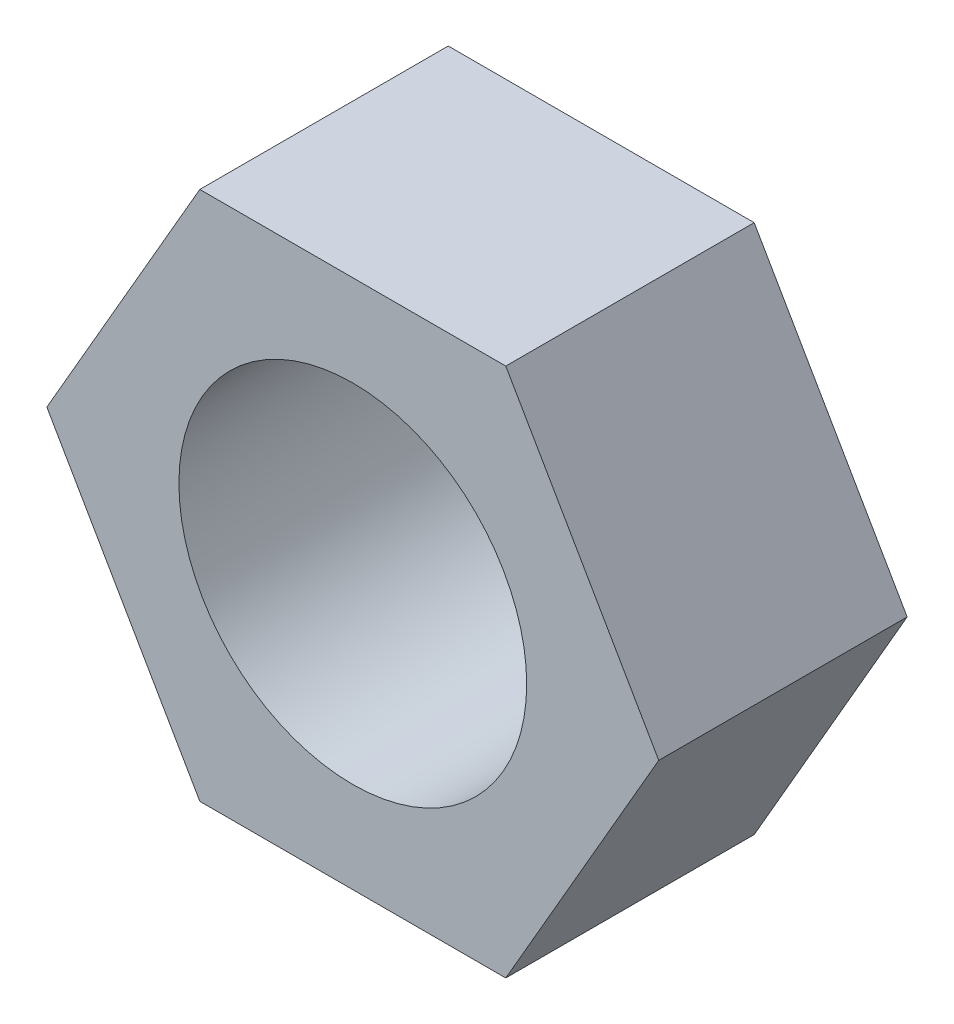
from build123d import *

# Parameters (mm, degrees)
BOSS_EXTRUDE1_DEPTH    = 15
M24_TAPPED_HOLE1_D     = 21
M24_TAPPED_HOLE1_DEPTH = 57
M24_TAPPED_HOLE1_TIP   = 6.3090365


with BuildPart() as part:
    # Sketch1 → Boss-Extrude1 (new body)
    with BuildSketch(Plane.XY):
        Polygon((18.475208614, 0), (9.237604307, 16), (-9.237604307, 16), (-18.475208614, 0), (-9.237604307, -16), (9.237604307, -16), align=None)
    extrude(amount=BOSS_EXTRUDE1_DEPTH)

    # M24 Tapped Hole1
    with Locations(Plane.XY.offset(15)):
        with Locations((0, 0)):
            Hole(M24_TAPPED_HOLE1_D / 2, depth=M24_TAPPED_HOLE1_DEPTH)
            with Locations((0, 0, -(M24_TAPPED_HOLE1_DEPTH + M24_TAPPED_HOLE1_TIP / 2))):  # 118° drill point
                Cone(0, M24_TAPPED_HOLE1_D / 2, M24_TAPPED_HOLE1_TIP, mode=Mode.SUBTRACT)


solid = part.part
